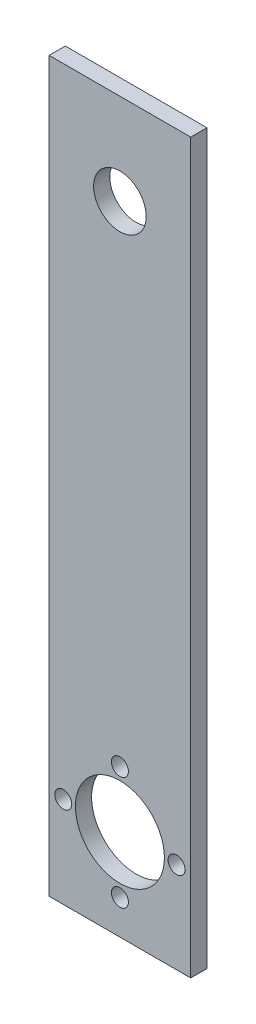
SolidWorks part; units mm, degrees
material "304"
ref_plane "Front Plane" through (0, 0, 0) normal (0, 0, 1) x (1, 0, 0)
ref_plane "Top Plane" through (0, 0, 0) normal (0, 1, 0) x (1, 0, 0)
ref_plane "Right Plane" through (0, 0, 0) normal (1, 0, 0) x (0, 0, -1)
sketch "Sketch1" plane through (0, 0, 0) normal (0, 0, 1) x (1, 0, 0)
  line L0 (17.5, -90) -> (72.0689, -90) construction
  line L1 (0, 0) -> (35, 0)
  line L2 (0, 0) -> (0, -180)
  line L3 (0, -180) -> (35, -180)
  line L4 (35, 0) -> (35, -180)
  line L5 (0, 0) -> (35, -180) construction
  line L6 (0, -180) -> (35, 0) construction
  circle A0 centre (17.5, -22.5) radius 6.5
  circle A1 centre (17.5, -157.5) radius 11
  point P6 (17.5, -90)
  dimension "D3" = 135
  dimension "D4" = 13
  dimension "D5" = 22
  dimension "D1" = 35
  dimension "D2" = 180
extrude "Boss-Extrude1" add sketch "Sketch1" along normal blind 4
sketch "Sketch2" plane through (0, 0, 4) normal (0, 0, 1) x (1, 0, 0)
  circle A0 centre (17.5, -157.5) radius 14 construction
  circle A1 centre (3.5, -157.5) radius 2.1
  circle A2 centre (17.5, -143.5) radius 2.1
  circle A3 centre (31.5, -157.5) radius 2.1
  circle A4 centre (17.5, -171.5) radius 2.1
  dimension "D1" = 28
  dimension "D2" = 4.2
extrude "Cut-Extrude2" cut sketch "Sketch2" against normal blind 10
